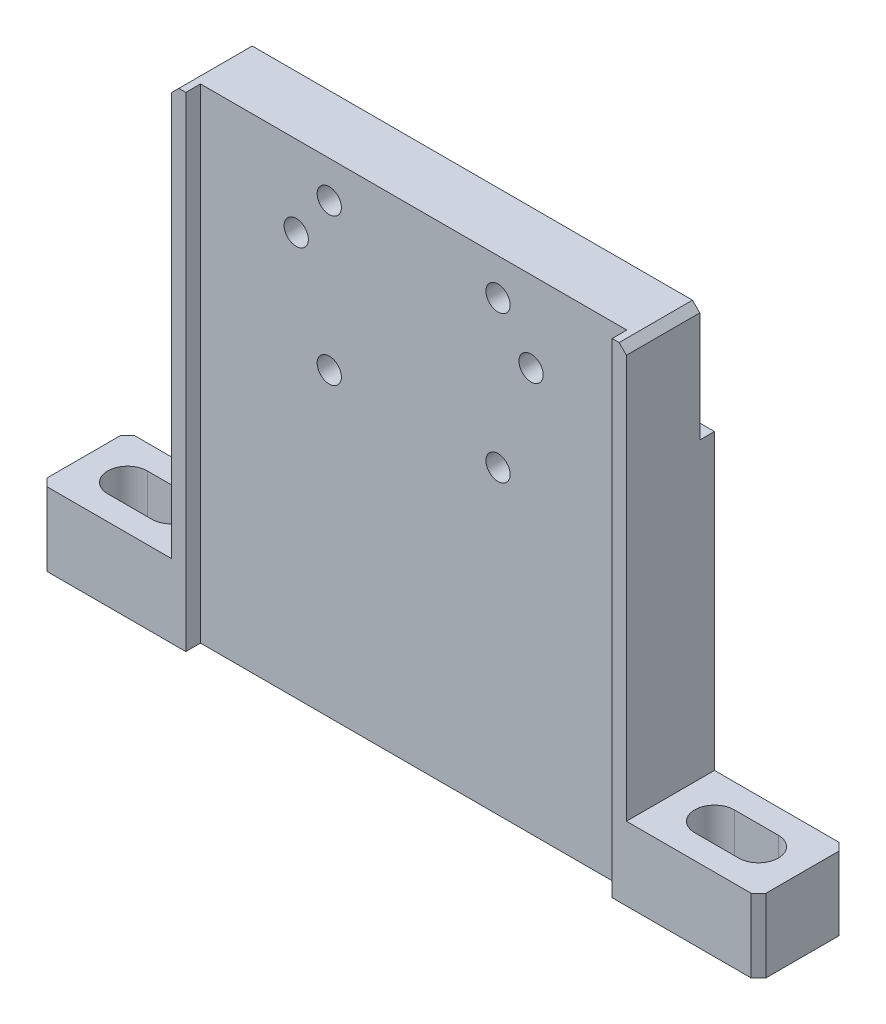
from build123d import *

# Parameters (mm, degrees)
SKETCH_1_W          = 62
SKETCH_1_H          = 66
EXTRUDE_1_DEPTH     = 6
SKETCH_3_W          = 58.1
SKETCH_3_H          = 113.69115984
CUT_EXTRUDE_1_DEPTH = 2
HOLE_WIZARD_M4_1_D  = 3.3
HOLE_WIZARD_M4_2_D  = 3.3
SKETCH_14_W         = 98
SKETCH_14_H         = 12
EXTRUDE_3_DEPTH     = 10
CUT_EXTRUDE_2_DEPTH = 75.652528423
SKETCH_16_W         = 58.1
SKETCH_16_H         = 41.285826149
CUT_EXTRUDE_3_DEPTH = 2
SKETCH_17_W         = 126.235416792
SKETCH_17_H         = 53.479043567
CUT_EXTRUDE_4_DEPTH = 2
CHAMFER_1_SIZE      = 1
CHAMFER_2_SIZE      = 1


with BuildPart() as part:
    # 草图1 → 凸台-拉伸1 (new, symmetric)
    with BuildSketch(Plane.XY):
        Rectangle(SKETCH_1_W, SKETCH_1_H)
    extrude(amount=EXTRUDE_1_DEPTH, both=True)

    # 草图3 → 切除-拉伸1 (cut)
    with BuildSketch(Plane.XY.offset(6)):
        Rectangle(SKETCH_3_W, SKETCH_3_H)
    extrude(amount=-CUT_EXTRUDE_1_DEPTH, mode=Mode.SUBTRACT)

    # M4 螺纹孔1 (through all)
    with Locations(Plane.XY.offset(4)):
        with Locations((-11.5, 28), (11.5, 28), (-11.5, 8), (11.5, 8)):
            Hole(HOLE_WIZARD_M4_1_D / 2)

    # M4 螺纹孔2 (through all)
    with Locations(Plane(origin=(0, 0, -6), x_dir=(-1, 0, 0), z_dir=(0, 0, -1))):
        with Locations((-16, 22), (16, 22)):
            Hole(HOLE_WIZARD_M4_2_D / 2)

    # 草图14 → 凸台-拉伸3 (add)
    with BuildSketch(Plane.XZ.offset(33)):
        Rectangle(SKETCH_14_W, SKETCH_14_H)
    extrude(amount=-EXTRUDE_3_DEPTH)

    # 草图15 → 切除-拉伸2 (cut, through all)
    with BuildSketch(Plane(origin=(0, -23, 0), x_dir=(1, 0, 0), z_dir=(0, 1, 0))):
        with BuildLine():
            Line((-43, 2.7), (-37, 2.7))
            ThreePointArc((-37, 2.7), (-34.3, 0), (-37, -2.7))
            Line((-37, -2.7), (-43, -2.7))
            ThreePointArc((-43, -2.7), (-45.7, 0), (-43, 2.7))
        make_face()
    cut_extrude_2 = extrude(amount=-CUT_EXTRUDE_2_DEPTH, mode=Mode.SUBTRACT)

    # 镜向1: 切除-拉伸2 across plane
    add(cut_extrude_2.mirror(Plane(origin=(0, 0, 0), x_dir=(0, 0, 1), z_dir=(1, 0, 0))), mode=Mode.SUBTRACT)

    # 草图16 → 切除-拉伸3 (cut)
    with BuildSketch(Plane.XY.offset(6)):
        with Locations((0, -39.137864824)):
            Rectangle(SKETCH_16_W, SKETCH_16_H)
    extrude(amount=-CUT_EXTRUDE_3_DEPTH, mode=Mode.SUBTRACT)

    # 草图17 → 切除-拉伸4 (cut)
    with BuildSketch(Plane(origin=(0, 0, -6), x_dir=(-1, 0, 0), z_dir=(0, 0, -1))):
        with Locations((-8.783621981, 43.739521784)):
            Rectangle(SKETCH_17_W, SKETCH_17_H)
    extrude(amount=-CUT_EXTRUDE_4_DEPTH, mode=Mode.SUBTRACT)

    # 倒角1
    chamfer_1_edges = [part.edges().sort_by_distance(p)[0] for p in [
        (49, -28, -6),
        (-49, -28, 6),
        (49, -28, 6),
        (-49, -28, -6),
    ]]
    chamfer(chamfer_1_edges, length=CHAMFER_1_SIZE)

    # 倒角2
    chamfer_2_edges = [part.edges().sort_by_distance(p)[0] for p in [
        (-31, 33, 1),
        (31, 33, 1),
    ]]
    chamfer(chamfer_2_edges, length=CHAMFER_2_SIZE)


solid = part.part
